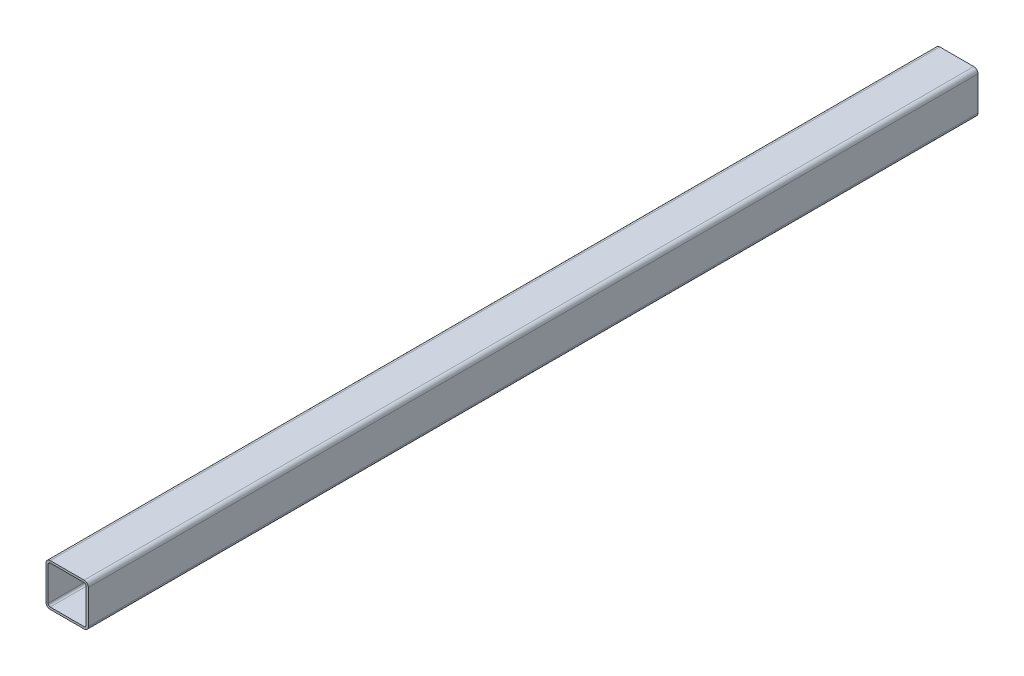
from build123d import *

# Parameters (mm, degrees)
BOSS_EXTRUDE_1_DEPTH = 1050


with BuildPart() as part:
    # Sketch 1 → Boss-Extrude 1 (new, symmetric)
    with BuildSketch(Plane.XY):
        with BuildLine():
            Line((0, 50), (-40, 50))
            ThreePointArc((-40, 50), (-47.071067812, 47.071067812), (-50, 40))
            Line((-50, 40), (-50, 0))
            Line((-50, 0), (-50, -40))
            ThreePointArc((-50, -40), (-47.071067812, -47.071067812), (-40, -50))
            Line((-40, -50), (40, -50))
            ThreePointArc((40, -50), (47.071067812, -47.071067812), (50, -40))
            Line((50, -40), (50, 0))
            Line((50, 0), (50, 40))
            ThreePointArc((50, 40), (47.071067812, 47.071067812), (40, 50))
            Line((40, 50), (0, 50))
        make_face()
        with BuildLine():
            Line((0, 45), (-40, 45))
            ThreePointArc((-40, 45), (-43.535533906, 43.535533906), (-45, 40))
            Line((-45, 40), (-45, 0))
            Line((-45, 0), (-45, -40))
            ThreePointArc((-45, -40), (-43.535533906, -43.535533906), (-40, -45))
            Line((-40, -45), (40, -45))
            ThreePointArc((40, -45), (43.535533906, -43.535533906), (45, -40))
            Line((45, -40), (45, 0))
            Line((45, 0), (45, 40))
            ThreePointArc((45, 40), (43.535533906, 43.535533906), (40, 45))
            Line((40, 45), (0, 45))
        make_face(mode=Mode.SUBTRACT)
    extrude(amount=BOSS_EXTRUDE_1_DEPTH, both=True)


solid = part.part
